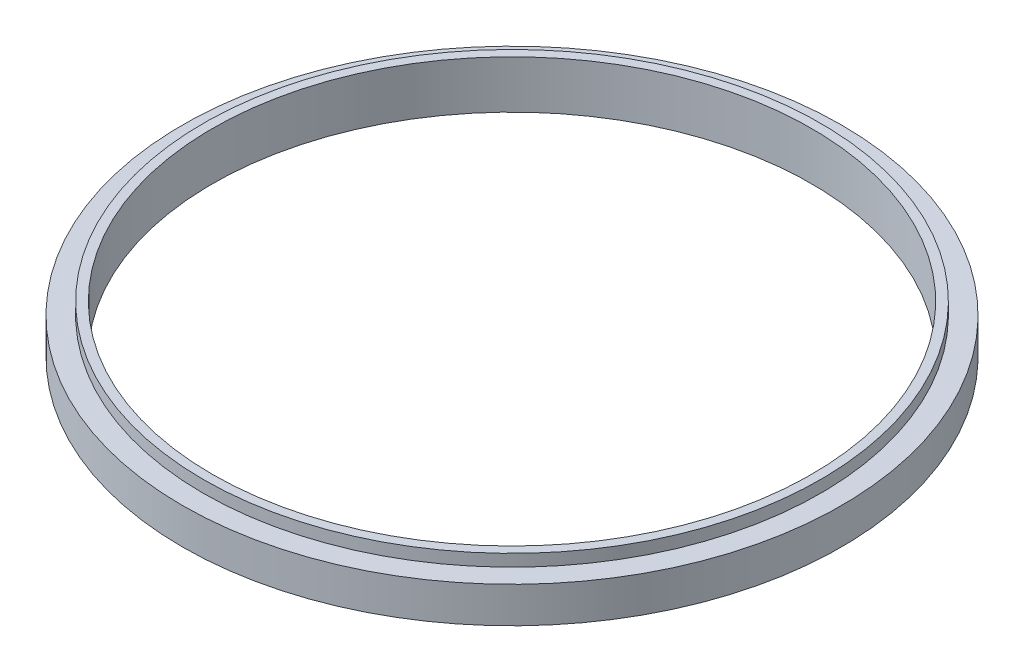
from build123d import *

# Parameters (mm, degrees)
SKETCH1_R           = 55
SKETCH1_R_2         = 50
BOSS_EXTRUDE1_DEPTH = 6
SKETCH2_R           = 51.5
SKETCH2_R_2         = 50
BOSS_EXTRUDE2_DEPTH = 2


with BuildPart() as part:
    # Sketch1 → Boss-Extrude1 (new body)
    with BuildSketch(Plane(origin=(0, 0, 0), x_dir=(1, 0, 0), z_dir=(0, 1, 0))):
        with Locations(Location((0, 0, 0), (0, 0, 270))):
            Circle(SKETCH1_R)
        with Locations(Location((0, 0, 0), (0, 0, 270))):
            Circle(SKETCH1_R_2, mode=Mode.SUBTRACT)
    extrude(amount=BOSS_EXTRUDE1_DEPTH)

    # Sketch2 → Boss-Extrude2 (add)
    with BuildSketch(Plane(origin=(0, 6, 0), x_dir=(1, 0, 0), z_dir=(0, 1, 0))):
        with Locations(Location((0, 0, 0), (0, 0, 270))):
            Circle(SKETCH2_R)
        with Locations(Location((0, 0, 0), (0, 0, 270))):
            Circle(SKETCH2_R_2, mode=Mode.SUBTRACT)
    extrude(amount=BOSS_EXTRUDE2_DEPTH)


solid = part.part
